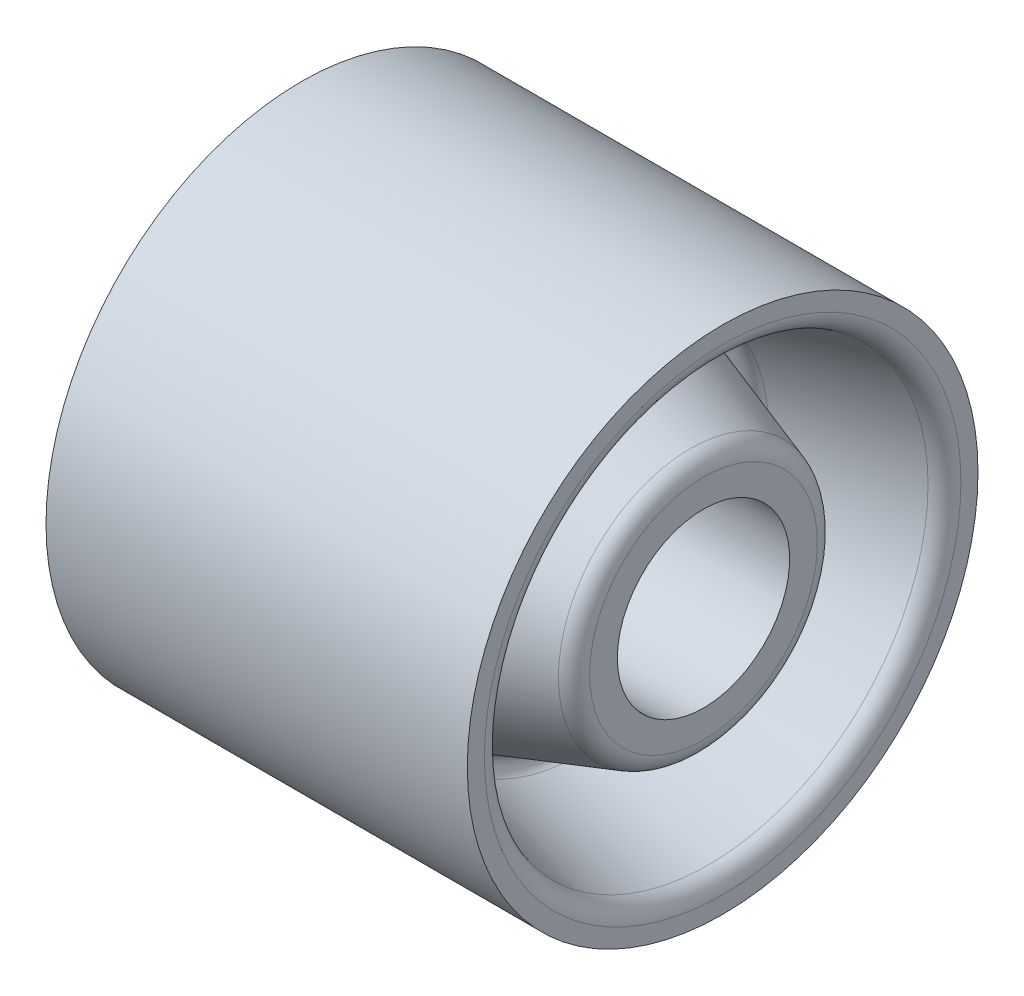
SolidWorks part; units mm, degrees
ref_plane "Front Plane" through (0, 0, 0) normal (0, 0, 1) x (1, 0, 0)
ref_plane "Top Plane" through (0, 0, 0) normal (0, 1, 0) x (1, 0, 0)
ref_plane "Right Plane" through (0, 0, 0) normal (1, 0, 0) x (0, 0, -1)
sketch "Sketch1" plane through (0, 0, 0) normal (0, 0, 1) x (1, 0, 0)
  line L0 (0, 0) -> (66, 0) construction
  line L1 (0, 40) -> (66, 40)
  line L2 (66, 40) -> (66, 37.3214)
  line L3 (63.7529, 34.4174) -> (43.9067, 29.2721)
  line L4 (43.8088, 26.3971) -> (60.9487, 20.6838)
  line L5 (63, 17.8377) -> (63, 13.5)
  line L6 (63, 13.5) -> (3, 13.5)
  line L7 (3, 13.5) -> (3, 17.8377)
  line L8 (5.0513, 20.6838) -> (22.1912, 26.3971)
  line L9 (22.0933, 29.2721) -> (2.2471, 34.4174)
  line L10 (0, 37.3214) -> (0, 40)
  line L11 (44.2831, 27.8201) -> (21.7169, 27.8201) construction
  arc A0 (22.1912, 26.3971) -> (22.0933, 29.2721) centre (21.7169, 27.8201) ccw
  arc A1 (43.9067, 29.2721) -> (43.8088, 26.3971) centre (44.2831, 27.8201) ccw
  arc A2 (60.9487, 20.6838) -> (63, 17.8377) centre (60, 17.8377) cw
  arc A3 (3, 17.8377) -> (5.0513, 20.6838) centre (6, 17.8377) cw
  arc A4 (2.2471, 34.4174) -> (0, 37.3214) centre (3, 37.3214) cw
  arc A5 (66, 37.3214) -> (63.7529, 34.4174) centre (63, 37.3214) cw
  point P13 (33, 27.8201)
  point P14 (33, 0)
  point P18 (27, 28)
  point P21 (39, 28)
  point P24 (63, 20)
  point P27 (3, 20)
  point P30 (0, 35)
  point P33 (66, 35)
  dimension "D11" = 1.5
  dimension "D12" = 3
  dimension "D1" = 66
  dimension "D2" = 12
  dimension "D3" = 66
  dimension "D4" = 60
  dimension "D5" = 20
  dimension "D6" = 40
  dimension "D7" = 35
  dimension "D8" = 13.5
  dimension "D9" = 28
  dimension "D10" = 3
revolve "Revolve1" add sketch "Sketch1" angle 360 about L0
